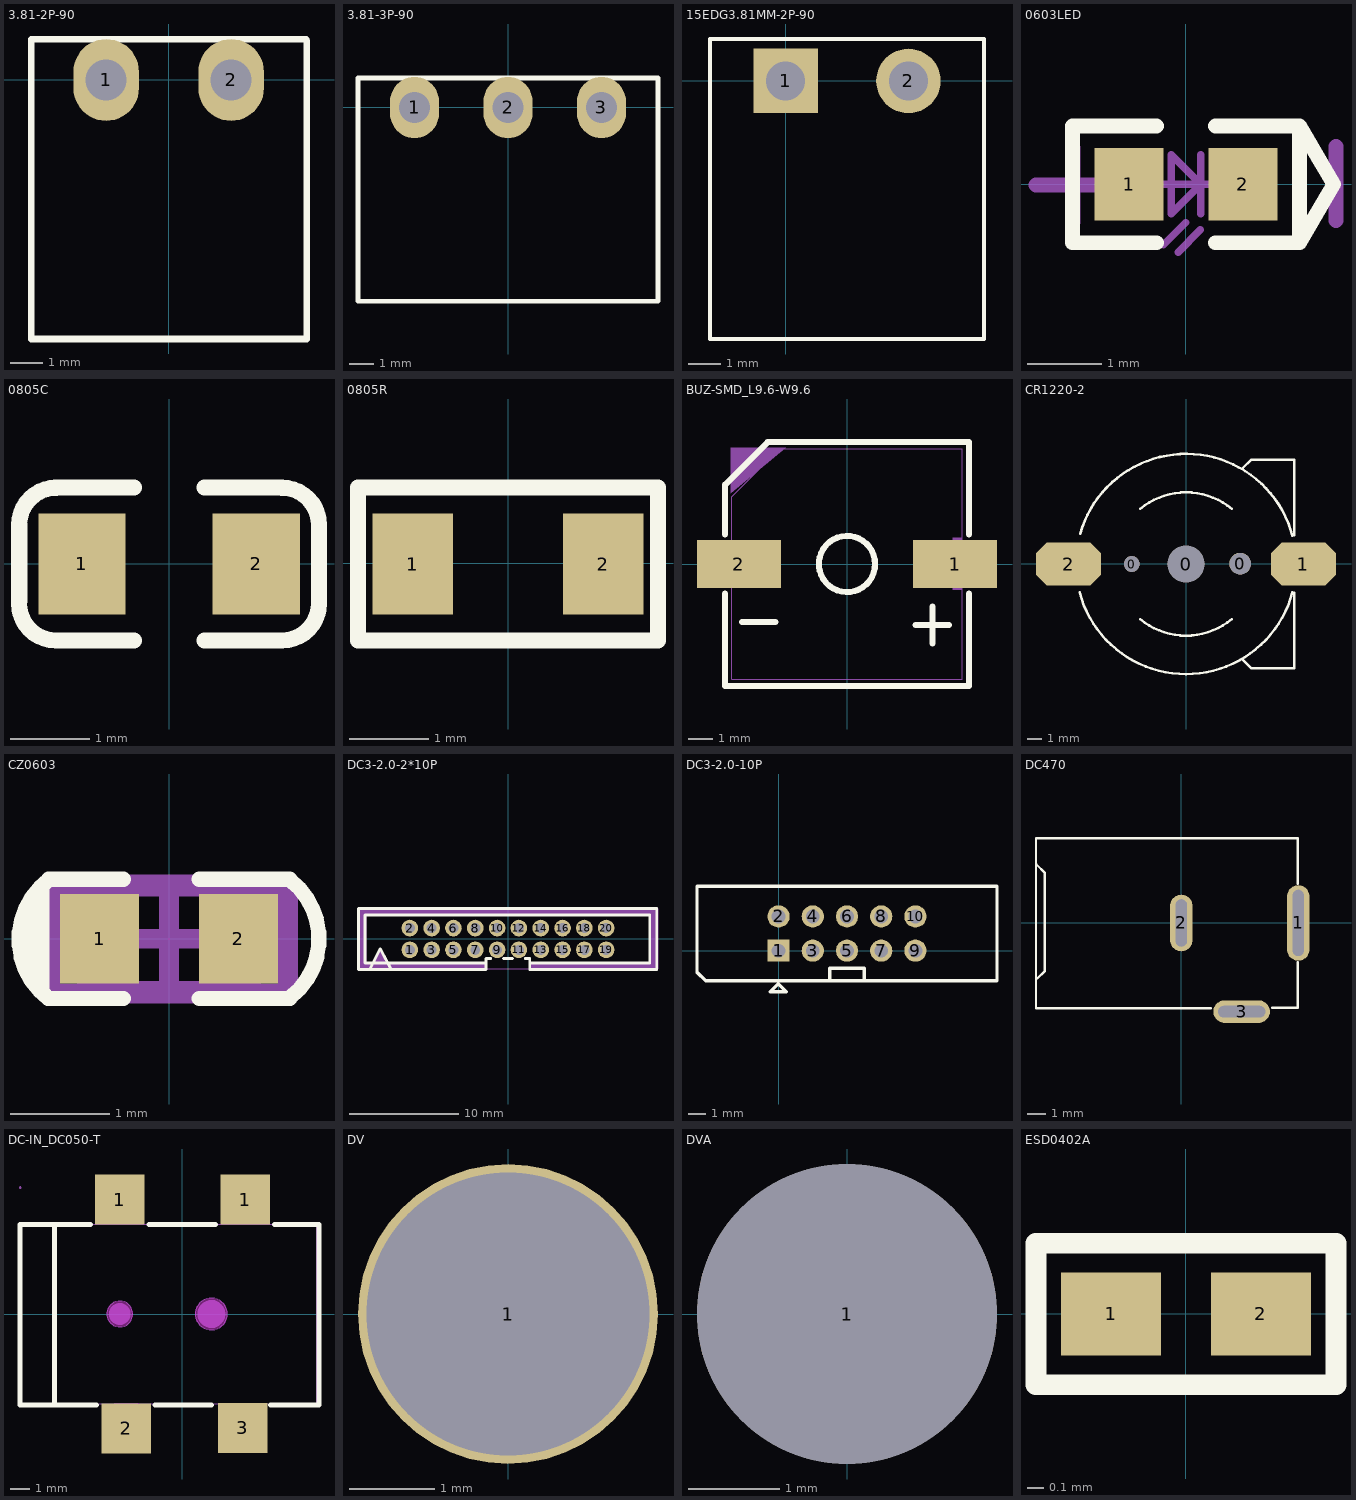
[diagram p0: the footprints below, top view; thin cyan lines are the x and y axes]
# Altium footprint library MISC82162-2.PcbLib: 66 footprints (part 1 of 5)
Each footprint in its own frame and in the unit in brackets; x right, y up, seen from the top. Pads: shape width x height; smd on the part's side, far side on the other; paste and mask are expansions set on the pad; w line width, h text height; cw(c..) or ccw(c..) is an arc to the next point about the centre after c.

## 3.81-2P-90 [mm]
pads (2):
  oval 2x2.5 hole 1.25: 1(-1.905,0) 2(1.905,0)
Top Overlay:
  lines w0.2: 4.191,-7.9 -4.191,-7.9 -4.191,1.244 4.191,1.244 ; 4.21,-7.9 4.21,1.2

## 3.81-3P-90 [mm]
pads (3):
  oval 2x2.5 hole 1.25: 1(-3.81,0) 2(0,0) 3(3.81,0)
Top Overlay:
  lines w0.2: -6.115,-7.9 6.115,-7.9 6.115,1.2 -6.115,1.2 -6.115,-7.9

## 15EDG3.81MM-2P-90 [mm]
pads (2):
  rect 2x2 / inner round 2 / far side rect 2x2 hole 1.2: 1(0,0)
  round 2 hole 1.2: 2(3.81,0)
Top Overlay:
  lines w0.127: -2.34,-8 -2.34,1.3 6.15,1.3 6.15,-8 -2.34,-8

## 0603LED [mm]
pads (2):
  rect 0.93x0.98 smd: 1(-0.77,0) 2(0.77,0)
Top Overlay:
  lines w0.2: -0.4,-0.79 -1.535,-0.79 -1.535,0.79 -0.4,0.79 ; 0.4,-0.79 1.535,-0.79 ; 0.4,0.79 1.535,0.79 ; 1.535,-0.79 1.535,0.79 ; 1.535,-0.79 2,0 1.535,0.79
Mechanical 13:
  lines w0.1: -0.4,0 0.4,0 ; -0.305,-0.817 -0.005,-0.517 ; -0.105,-0.917 0.195,-0.617 ; 0.2,-0.4 0.2,0.4 ; -0.2,-0.4 0.2,0 -0.2,0.4 -0.2,-0.4
Mechanical 15:
  lines w0.203: -2.03,-0.01 -1.03,-0.01 ; -1.53,-0.51 -1.53,0.49 ; 2.03,-0.49 2.03,0.51

## 0805C [mm]
pads (2):
  rect 1.1x1.27 smd: 1(-1.1,0) 2(1.1,0)
Top Overlay:
  lines w0.203: -1.895,-0.498 ccw(c-1.427,-0.498) -1.427,-0.965 ; -1.892,-0.47 -1.892,0.47 ; -1.892,0.495 cw(c-1.425,0.495) -1.425,0.963 ; -1.438,0.965 -0.444,0.965 ; -1.402,-0.965 -0.444,-0.965 ; 0.445,-0.965 1.413,-0.965 ; 0.445,0.965 1.412,0.965 ; 1.425,-0.965 ccw(c1.425,-0.498) 1.892,-0.498 ; 1.425,0.963 cw(c1.425,0.495) 1.892,0.495 ; 1.892,-0.472 1.892,0.47

## 0805R [mil]
pads (2):
  rect 40x50 smd: 1(-47.28,-0.31) 2(47.21,-0.31)
Top Overlay:
  lines w8: -74.53,-38.31 74.47,-38.31 74.47,37.69 -74.53,37.69 -74.53,-38.31

## BUZ-SMD_L9.6-W9.6 [mm]
pads (2):
  rect 3.5x2 smd: 1(4.5,0) 2(-4.5,0)
Top Overlay:
  circle w0.254: c0.001,0 r1.171
  lines w0.254: -5.08,-1.232 -5.08,-5.08 5.08,-5.08 5.08,-1.231 ; -5.08,1.232 -5.08,3.302 -3.302,5.08 5.08,5.08 5.08,1.231 ; -4.381,-2.413 -2.984,-2.413 ; 2.858,-2.54 4.255,-2.54 ; 3.556,-3.302 3.556,-1.778
Mechanical 6:
  region: -2.55,4.85 -4.85,4.85 -4.85,2.95
  region: -5.508,0.191 -3.349,0.191 -3.349,-0.191 -5.508,-0.191
  region: 4.41,-1.07 4.41,1.089 4.791,1.089 4.791,-1.07
  region: 3.492,0.191 5.651,0.191 5.651,-0.191 3.492,-0.191
Mechanical 15:
  region: -3.3,-0.75 -5,-0.75 -5,0.75 -3.3,0.75
  region: 3.3,0.75 5,0.75 5,-0.75 3.3,-0.75
  lines w0.051: -4.8,-4.8 -4.8,2.8 -2.8,4.8 4.8,4.8 4.8,-4.8 -4.8,-4.8

## CR1220-2 [mm]
pads (5):
  round 1.1 hole 1.1: 0(-3.75,-0.012)
  round 2.54 hole 2.54: 0(0,-0.012)
  round 1.5 hole 1.5: 0(3.75,0.012)
  oct 4.5x3 smd: 1(8.128,-0.012) 2(-8.128,-0.012)
Top Overlay:
  lines w0.178: -7.363,-1.976 ccw(c0,-0.012) 0,-7.632 ccw(c0,-0.012) 7.363,-1.976 ; -7.327,2.081 cw(c0,-0.012) 7.363,1.951 ; -3.172,-3.825 ccw(c0,-0.012) 3.169,-3.827 ; -3.172,3.8 cw(c0,-0.012) 3.175,3.797 ; 3.9,-6.613 4.5,-7.213 7.5,-7.213 7.5,-2.013 ; 3.925,6.612 4.5,7.187 7.5,7.187 7.5,1.988

## CZ0603 [mm]
pads (2):
  rect 0.8x0.9 smd: 1(-0.7,0) 2(0.7,0)
Top Overlay:
  lines w0.127: -1.27,-0.547 -1.27,0.549
  lines w0.152: -1.27,-0.547 -1.217,-0.6 -0.457,-0.6 ; -1.218,-0.599 cw(c-0.762,-0.005) -1.213,0.594 ; -1.213,0.6 -0.457,0.6 ; 0.305,-0.6 1.219,-0.6 ; 0.305,0.6 1.216,0.6 ; 1.217,-0.595 ccw(c0.762,0) 1.216,0.596
  lines w0.203: -1.372,-0.305 -1.372,0.356
Mechanical 13:
  lines w0.1: -0.875,-0.475 -0.875,0.475 0.875,0.475 0.875,-0.475 -0.875,-0.475
Mechanical 15:
  lines w0.2: -0.475,0 0.475,0 ; 0,-0.475 0,0.475 ; -1.2,-0.55 -1.2,0.55 1.2,0.55 1.2,-0.55 -1.2,-0.55

## DC3-2.0-2*10P [mil]
pads (20):
  round 60 hole 36: 1(-354.35,-39.37) 2(-354.35,39.37) 3(-275.55,-39.37) 4(-275.59,39.37) 5(-196.85,-39.37) 6(-196.85,39.37) 7(-118.15,-39.37) 8(-118.11,39.37) 9(-39.35,-39.37) 10(-39.37,39.37) 11(39.35,-39.37) 12(39.37,39.37) 13(118.15,-39.37) 14(118.11,39.37) 15(196.85,-39.37) 16(196.85,39.37) 17(275.55,-39.37) 18(275.59,39.37) 19(354.35,-39.37) 20(354.33,39.37)
Top Overlay:
  lines w10: -539.95,-110.07 -539.95,110.41 ; -539.82,-110.19 -79.19,-110.19 -79.19,-106.25 -79.19,-70.82 -62.49,-70.82 ; -537.85,110.29 536.95,110.29 536.95,-110.19 ; -500.45,86.66 511.36,86.66 511.36,-86.56 82.23,-86.56 ; -496.55,-106.25 -461.08,-35.38 -421.71,-110.19 ; -496.51,86.66 -516.2,86.66 -516.2,-86.56 -79.19,-86.56 ; -16.21,-70.82 16.21,-70.82 ; 62.49,-70.82 78.29,-70.82 78.29,-98.38 78.29,-110.19 534.98,-110.19
Mechanical 6:
  region: -492.13,-88.58 -433.07,-88.58 -462.6,-39.37
  region: -541.34,108.27 541.34,108.27 541.34,88.58 -511.81,88.58
  region: 541.34,-88.58 541.34,108.27 511.81,108.27 511.81,-88.58
  region: -541.34,-88.58 -541.34,108.27 -511.81,108.27 -511.81,-88.58
  region: 78.74,-108.27 78.74,-88.58 541.34,-88.58 541.34,-108.27
  region: -541.34,-108.27 -541.34,-88.58 -78.74,-88.58 -78.74,-108.27
Mechanical 15:
  region: -364.19,-29.53 -344.51,-29.53 -344.51,-49.21 -364.19,-49.21
  region: -364.19,49.21 -344.51,49.21 -344.51,29.53 -364.19,29.53
  region: -285.39,-29.53 -265.71,-29.53 -265.71,-49.21 -285.39,-49.21
  region: -285.43,49.21 -265.75,49.21 -265.75,29.53 -285.43,29.53
  region: -206.69,-29.53 -187.01,-29.53 -187.01,-49.21 -206.69,-49.21
  region: -206.69,49.21 -187.01,49.21 -187.01,29.53 -206.69,29.53
  region: -127.99,-29.53 -108.31,-29.53 -108.31,-49.21 -127.99,-49.21
  region: -127.95,49.21 -108.27,49.21 -108.27,29.53 -127.95,29.53
  region: -49.19,-29.53 -29.51,-29.53 -29.51,-49.21 -49.19,-49.21
  region: -49.21,49.21 -29.53,49.21 -29.53,29.53 -49.21,29.53
  region: 29.51,-29.53 49.19,-29.53 49.19,-49.21 29.51,-49.21
  region: 29.53,49.21 49.21,49.21 49.21,29.53 29.53,29.53
  region: 108.31,-29.53 127.99,-29.53 127.99,-49.21 108.31,-49.21
  region: 108.27,49.21 127.95,49.21 127.95,29.53 108.27,29.53
  region: 187.01,-29.53 206.69,-29.53 206.69,-49.21 187.01,-49.21
  region: 187.01,49.21 206.69,49.21 206.69,29.53 187.01,29.53
  region: 265.71,-29.53 285.39,-29.53 285.39,-49.21 265.71,-49.21
  region: 265.75,49.21 285.43,49.21 285.43,29.53 265.75,29.53
  region: 344.51,-29.53 364.19,-29.53 364.19,-49.21 344.51,-49.21
  region: 344.49,49.21 364.17,49.21 364.17,29.53 344.49,29.53
  region: -535.04,-108.27 -535.04,-107.29 -536.42,-105.91 -538.38,-105.91 -539.76,-107.29 -539.76,-108.27 -539.76,-109.25 -538.38,-110.63 -536.42,-110.63 -535.04,-109.25 -535.04,-108.27
  lines w2: -537.4,-108.27 537.4,-108.27 537.4,108.27 -537.4,108.27 -537.4,-108.27

## DC3-2.0-10P [mm]
pads (10):
  rect 1.3x1.3 hole 0.8: 1(0,0)
  round 1.3 hole 0.8: 2(0,2) 3(2,0) 4(2,2) 5(4,0) 6(4,2) 7(6,0) 8(6,2) 9(8,0) 10(8,2)
Top Overlay:
  lines w0.2: -0.013,-1.94 0.458,-2.411 -0.483,-2.411 -0.011,-1.939
  lines w0.203: 3,-1.77 3,-1.02 5,-1.02 5,-1.77 ; 12.7,-1.77 -4.262,-1.77 -4.77,-1.262 -4.77,3.77 12.77,3.77 12.77,-1.77

## DC470 [mm]
pads (3):
  oval 1.2x4 hole 0.6 slot 3.5 at 90 deg: 1(6.2,0)
  oval 1.2x3 hole 0.6 slot 2.5 at 90 deg: 2(0,0)
  oval 3x1.2 hole 0.6 slot 2.5 at 0 deg: 3(3.2,-4.7)
Top Overlay:
  lines w0.127: -7.7,-4.52 1.57,-4.52 ; -7.7,-4.5 -7.7,4.5 6.18,4.5 6.18,2.08 ; -7.69,3.11 -7.23,2.65 -7.23,-2.54 -7.63,-2.94 ; 4.83,-4.5 6.18,-4.5 6.18,-2.08

## DC-IN_DC050-T [mm]
pads (4):
  rect 2.5x2.5 smd paste+0 mask+0.05: 1(-3.15,5.75) 1(3.15,5.75) 2(-2.828,-5.75) 3(3.026,-5.725)
Top Overlay:
  lines w0.254: -8.15,-4.572 -4.331,-4.572 ; -8.15,-4.5 -8.15,4.5 -7.112,4.5 -4.631,4.5 ; -6.428,-4.572 -6.428,4.5 ; -1.669,4.5 1.669,4.5 ; -1.369,-4.572 1.469,-4.572 ; 4.431,-4.572 6.858,-4.572 6.858,4.5 4.631,4.5
Keep-Out Layer:
  board cut-out: 2.25,0 2.25,0.105 2.195,0.309 2.09,0.491 1.941,0.64 1.759,0.746 1.555,0.8 1.345,0.8 1.141,0.746 0.959,0.64 0.81,0.491 0.704,0.309 0.65,0.105 0.65,0 0.65,-0.105 0.704,-0.309 0.81,-0.491 0.959,-0.64 1.141,-0.745 1.345,-0.8 1.555,-0.8 1.759,-0.745 1.941,-0.64 2.09,-0.491 2.195,-0.309 2.25,-0.105
  board cut-out: -2.5,0 -2.5,0.086 -2.544,0.251 -2.63,0.399 -2.751,0.52 -2.899,0.606 -3.064,0.65 -3.236,0.65 -3.401,0.606 -3.549,0.52 -3.67,0.399 -3.756,0.251 -3.8,0.086 -3.8,0 -3.8,-0.085 -3.756,-0.251 -3.67,-0.399 -3.549,-0.52 -3.401,-0.606 -3.236,-0.65 -3.064,-0.65 -2.899,-0.606 -2.751,-0.52 -2.63,-0.399 -2.544,-0.251 -2.5,-0.085
Mechanical 1:
  circle w0.005: c1.45,0 r0.8
  circle w0.005: c-3.15,0 r0.65
Mechanical 6:
  circle w0.7: c1.45,0 r0.35
  circle w0.55: c-3.15,0 r0.275
Mechanical 15:
  region: 2.276,-6.345 2.276,-4.495 3.776,-4.495 3.776,-6.345
  region: 2.4,4.495 2.4,6.345 3.9,6.345 3.9,4.495
  region: -3.428,-6.345 -3.428,-4.495 -2.228,-4.495 -2.228,-6.345
  region: -3.75,4.495 -3.75,6.345 -2.55,6.345 -2.55,4.495
  region: -8.09,6.345 -8.09,6.37 -8.125,6.405 -8.175,6.405 -8.21,6.37 -8.21,6.345 -8.21,6.32 -8.175,6.285 -8.125,6.285 -8.09,6.32
  lines w0.051: -8.15,-4.5 6.75,-4.5 6.75,4.5 -8.15,4.5 -8.15,-4.5
Multi-Layer:
  pour cut-out: 2.25,0 2.25,0.105 2.195,0.309 2.09,0.491 1.941,0.64 1.759,0.746 1.555,0.8 1.345,0.8 1.141,0.746 0.959,0.64 0.81,0.491 0.704,0.309 0.65,0.105 0.65,0 0.65,-0.105 0.704,-0.309 0.81,-0.491 0.959,-0.64 1.141,-0.745 1.345,-0.8 1.555,-0.8 1.759,-0.745 1.941,-0.64 2.09,-0.491 2.195,-0.309 2.25,-0.105
  pour cut-out: -2.5,0 -2.5,0.086 -2.544,0.251 -2.63,0.399 -2.751,0.52 -2.899,0.606 -3.064,0.65 -3.236,0.65 -3.401,0.606 -3.549,0.52 -3.67,0.399 -3.756,0.251 -3.8,0.086 -3.8,0 -3.8,-0.085 -3.756,-0.251 -3.67,-0.399 -3.549,-0.52 -3.401,-0.606 -3.236,-0.65 -3.064,-0.65 -2.899,-0.606 -2.751,-0.52 -2.63,-0.399 -2.544,-0.251 -2.5,-0.085

## DV [mm]
pads (1):
  round 3.5 hole 3.3: 1(0,0)

## DVA [mm]
pads (1):
  round 3.3 hole 3.3 unplated: 1(0,0)

## ESD0402A [mil]
pads (2):
  rect 24x20 smd: 1(-18,0) 2(18,0)
Top Overlay:
  lines w5: -36,-17 -36,17 36,17 36,16 36,-17 -36,-17